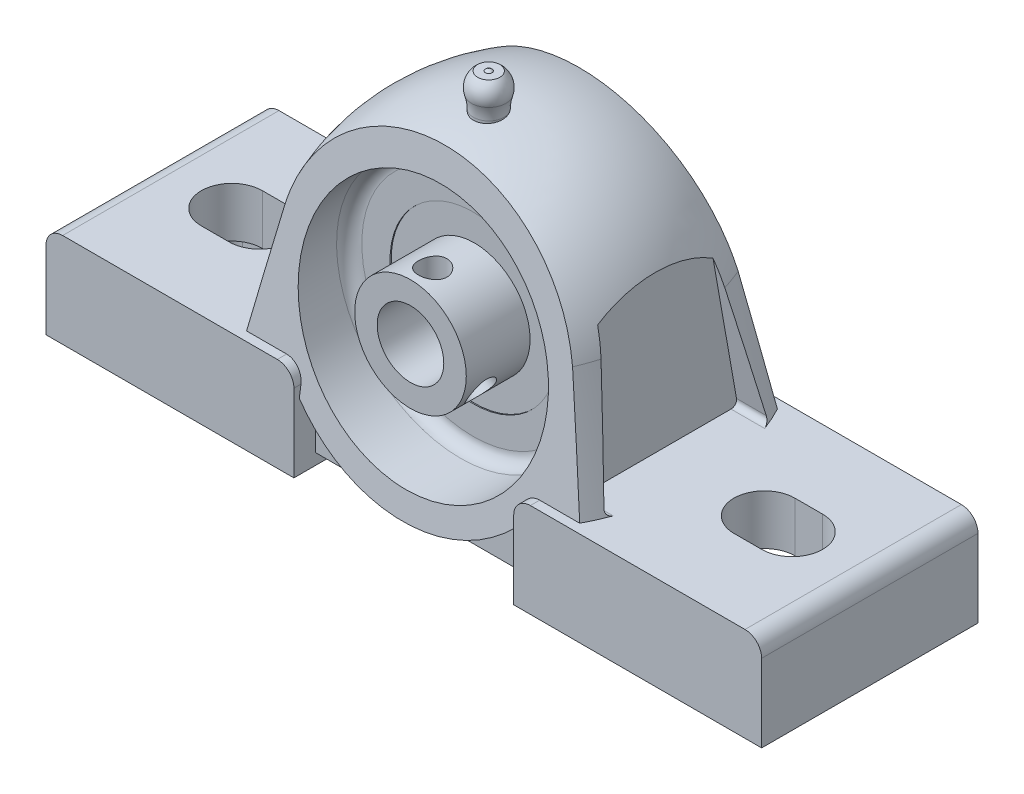
from build123d import *

# Parameters (mm, degrees)
BASE_EXTRUDE_DEPTH              = 78.25
CUT_EXTRUDE1_DEPTH              = 53.051467171
CUT_EXTRUDE1_DEPTH_BACK         = 53.051467171
SKETCH5_OUTSIDE_W               = 59.682
SKETCH5_OUTSIDE_H               = 80.692
BOSS_EXTRUDE4_REACH             = 57.711
BOSS_EXTRUDE4_DIRECTION_2_REACH = 57.711
BOSS_EXTRUDE1_DEPTH             = 19.5
BOSS_EXTRUDE1_DEPTH_BACK        = 19.5
CUT_EXTRUDE3_DEPTH              = 95.411036953
CUT_EXTRUDE4_DEPTH              = 7.99
CUT_EXTRUDE4_DRAFT              = -1
CUT_EXTRUDE4_PROFILE_2_DEPTH    = 7.99
CUT_EXTRUDE4_PROFILE_2_DRAFT    = -1
CIRPATTERN1_COUNT               = 9
SKETCH14_W                      = 31
SKETCH14_H                      = 4.06
SKETCH16_W                      = 2.567
SKETCH16_H                      = 6.26
SKETCH15_W                      = 0.1
SKETCH15_H                      = 5.32
CIRPATTERN2_COUNT               = 2
CIRPATTERN2_ANGLE               = 120
CUT_EXTRUDE5_START              = 25.83943
CUT_EXTRUDE5_DEPTH              = 12.56057
CUT_EXTRUDE6_START              = -38.4
CUT_EXTRUDE6_DEPTH              = 12.24096


with BuildPart() as part:
    # Sketch1 → Base-Extrude (new body)
    with BuildSketch(Plane(origin=(0, -28.2, 0), x_dir=(-1, 0, 0), z_dir=(0, 1, 0))):
        with BuildLine():
            Line((-33.636057661, 18.525), (33.636057661, 18.525))
            ThreePointArc((33.636057661, 18.525), (38.4, 0), (33.636057661, -18.525))
            Line((33.636057661, -18.525), (-33.636057661, -18.525))
            ThreePointArc((-33.636057661, -18.525), (-38.4, 0), (-33.636057661, 18.525))
        make_face()
    extrude(amount=BASE_EXTRUDE_DEPTH)

    # Cut-Sweep1: sweep along a path in Sketch3
    with BuildLine(Plane.XY) as cut_sweep1_path:
        Line((-38.4, -28.2), (-28.856466036, 7.676194886))
        ThreePointArc((-28.856466036, 7.676194886), (0, 29.86), (28.856466036, 7.676194886))
        Line((28.856466036, 7.676194886), (38.4, -28.2))
    # Sketch2 → Cut-Sweep1 (sweep, cut)
    with BuildSketch(Plane(origin=(0, -28.2, 0), x_dir=(-1, 0, 0), z_dir=(0, 1, 0))):
        with BuildLine():
            Line((-33.636057661, 18.525), (-116.65, 18.525))
            Line((-116.65, 18.525), (-116.65, -18.525))
            Line((-116.65, -18.525), (-33.636057661, -18.525))
            ThreePointArc((-33.636057661, -18.525), (-38.4, 0), (-33.636057661, 18.525))
        make_face()
    sweep(path=cut_sweep1_path.line, mode=Mode.SUBTRACT)

    # Sketch5 outside → Cut-Extrude1 (cut, two sides: drawn at the far end of the back side and taken through both)
    with BuildSketch(Plane(origin=(0, 0, 0), x_dir=(0, 0, -1), z_dir=(1, 0, 0)).offset(-CUT_EXTRUDE1_DEPTH_BACK)):
        with Locations((0, 0.83)):
            Rectangle(SKETCH5_OUTSIDE_W, SKETCH5_OUTSIDE_H)
        Polygon((11.7, 30.86), (18.525, -18.28), (15.6, -18.28), (15.6, -31.2), (-15.6, -31.2), (-15.6, -18.28), (-18.525, -18.28), (-11.7, 30.86), align=None, mode=Mode.SUBTRACT)
    extrude(amount=CUT_EXTRUDE1_DEPTH + CUT_EXTRUDE1_DEPTH_BACK, mode=Mode.SUBTRACT)

    # Sketch6 → Cut-Revolve2 (revolve, cut)
    with BuildSketch(Plane(origin=(0, 0, 0), x_dir=(0, 0, -1), z_dir=(1, 0, 0)), mode=Mode.PRIVATE) as cut_revolve2_sk:
        with BuildLine():
            Line((-22.725865299, 22.347619048), (-9.277190476, 22.347619048))
            ThreePointArc((-9.277190476, 22.347619048), (-7.666973648, 21.680645399), (-7, 20.070428571))
            Line((-7, 20.070428571), (-7, 18.734993995))
            ThreePointArc((-7, 18.734993995), (-6.071328156, 19.056205667), (-5.128, 19.331415261))
            Line((-5.128, 19.331415261), (-5.128, 22.347619048))
            Line((-5.128, 22.347619048), (-3.256, 22.347619048))
            Line((-3.256, 22.347619048), (-3.256, 19.733181801))
            ThreePointArc((-3.256, 19.733181801), (1.937389668, 19.905941859), (7, 18.734993995))
            Line((7, 18.734993995), (7, 20.070428571))
            ThreePointArc((7, 20.070428571), (7.666973648, 21.680645399), (9.277190476, 22.347619048))
            Line((9.277190476, 22.347619048), (22.725865299, 22.347619048))
            Line((22.725865299, 22.347619048), (25.829701277, 0))
            Line((25.829701277, 0), (-25.829701277, 0))
            Line((-25.829701277, 0), (-22.725865299, 22.347619048))
        make_face()
    revolve(cut_revolve2_sk.sketch.rotate(Axis((0, 0, 0), (0, 0, -1)), 180), axis=Axis((0, 0, 0), (0, 0, -1)), mode=Mode.SUBTRACT)

    # Sketch11 → Boss-Revolve1 (revolve)
    with BuildSketch(Plane.XY.offset(4.192)):
        with BuildLine():
            Line((0, 27.973774284), (0, 35.86))
            ThreePointArc((0, 35.86), (-0.328456711, 35.790107141), (-0.6, 35.592539267))
            Line((-0.6, 35.592539267), (-2, 35.592539267))
            ThreePointArc((-2, 35.592539267), (-3.100653507, 34.004684437), (-3.105555556, 32.072665525))
            ThreePointArc((-3.105555556, 32.072665525), (-2.83938828, 30.906746373), (-2.75, 29.714176785))
            Line((-2.75, 29.714176785), (-2.75, 27.973774284))
            Line((-2.75, 27.973774284), (0, 27.973774284))
        make_face()
    revolve(axis=Axis((0, 0, 4.192), (0, 1, 0)))

    # Boss-Extrude4: up to this plane
    boss_extrude4_end = Plane(origin=(-38.4, 30.86, -11.7), z_dir=(0, 0.137568371274657, -0.9904922731777558))
    # Sketch9 → Boss-Extrude4 (add, up to the surface)
    with BuildSketch(Plane.XY, mode=Mode.PRIVATE) as boss_extrude4_sk1:
        with BuildLine():
            Line((12.855258733, -18.28), (19.810146566, -18.28))
            ThreePointArc((19.810146566, -18.28), (0, -26.955524609), (-19.810146566, -18.28))
            Line((-19.810146566, -18.28), (-12.855258733, -18.28))
            ThreePointArc((-12.855258733, -18.28), (0, -22.347619048), (12.855258733, -18.28))
        make_face()
    boss_extrude4_tool1 = split(extrude(boss_extrude4_sk1.sketch, amount=-BOSS_EXTRUDE4_REACH, mode=Mode.PRIVATE), bisect_by=boss_extrude4_end, keep=Keep.BOTH, mode=Mode.PRIVATE)
    add(boss_extrude4_tool1.solids().sort_by_distance((0, -22.606339, 0))[0])

    # Boss-Extrude4 direction 2: up to this plane
    boss_extrude4_direction_2_end = Plane(origin=(-38.4, 30.86, 11.7), z_dir=(0, 0.137568371274657, 0.9904922731777558))
    # Sketch9 → Boss-Extrude4 direction 2 (add, up to the surface)
    with BuildSketch(Plane.XY, mode=Mode.PRIVATE) as boss_extrude4_direction_2_sk1:
        with BuildLine():
            Line((12.855258733, -18.28), (19.810146566, -18.28))
            ThreePointArc((19.810146566, -18.28), (0, -26.955524609), (-19.810146566, -18.28))
            Line((-19.810146566, -18.28), (-12.855258733, -18.28))
            ThreePointArc((-12.855258733, -18.28), (0, -22.347619048), (12.855258733, -18.28))
        make_face()
    boss_extrude4_direction_2_tool1 = split(extrude(boss_extrude4_direction_2_sk1.sketch, amount=BOSS_EXTRUDE4_DIRECTION_2_REACH, mode=Mode.PRIVATE), bisect_by=boss_extrude4_direction_2_end, keep=Keep.BOTH, mode=Mode.PRIVATE)
    add(boss_extrude4_direction_2_tool1.solids().sort_by_distance((0, -22.606339, 0))[0])

    # Sketch4 → Boss-Extrude1 (add, two sides: drawn at the far end of the back side and taken through both)
    with BuildSketch(Plane.XY.offset(-BOSS_EXTRUDE1_DEPTH_BACK)):
        with BuildLine():
            Line((22.810146566, -13.2), (61.5, -13.2))
            ThreePointArc((61.5, -13.2), (63.621320344, -14.078679656), (64.5, -16.2))
            Line((64.5, -16.2), (64.5, -30.2))
            Line((64.5, -30.2), (19.810146566, -30.2))
            Line((19.810146566, -30.2), (19.810146566, -16.2))
            ThreePointArc((19.810146566, -16.2), (20.688826222, -14.078679656), (22.810146566, -13.2))
        make_face()
        with BuildLine():
            Line((-61.5, -13.2), (-22.810146566, -13.2))
            ThreePointArc((-22.810146566, -13.2), (-20.688826222, -14.078679656), (-19.810146566, -16.2))
            Line((-19.810146566, -16.2), (-19.810146566, -30.2))
            Line((-19.810146566, -30.2), (-64.5, -30.2))
            Line((-64.5, -30.2), (-64.5, -16.2))
            ThreePointArc((-64.5, -16.2), (-63.621320344, -14.078679656), (-61.5, -13.2))
        make_face()
    extrude(amount=BOSS_EXTRUDE1_DEPTH + BOSS_EXTRUDE1_DEPTH_BACK)

    # Sketch7 → Cut-Extrude3 (cut, through all)
    with BuildSketch(Plane.XZ.offset(30.2)):
        with BuildLine():
            Line((-45.5, 5.5), (-50.5, 5.5))
            ThreePointArc((-50.5, 5.5), (-56, 0), (-50.5, -5.5))
            Line((-50.5, -5.5), (-45.5, -5.5))
            ThreePointArc((-45.5, -5.5), (-40, 0), (-45.5, 5.5))
        make_face()
        with BuildLine():
            Line((45.5, -5.5), (50.5, -5.5))
            ThreePointArc((50.5, -5.5), (56, 0), (50.5, 5.5))
            Line((50.5, 5.5), (45.5, 5.5))
            ThreePointArc((45.5, 5.5), (40, 0), (45.5, -5.5))
        make_face()
    extrude(amount=-CUT_EXTRUDE3_DEPTH, mode=Mode.SUBTRACT)


with BuildPart() as cut_extrude4_tool:
    # Sketch10 → Cut-Extrude4 (with draft: the straight prism first)
    with BuildSketch(Plane.XZ.offset(30.2)):
        with BuildLine():
            ThreePointArc((50.5, -10.73), (51.015492065, -9.485492065), (52.26, -8.97))
            Line((52.26, -8.97), (57.475, -8.97))
            ThreePointArc((57.475, -8.97), (58.719507935, -8.454507935), (59.235, -7.21))
            Line((59.235, -7.21), (59.235, 7.21))
            ThreePointArc((59.235, 7.21), (58.719507935, 8.454507935), (57.475, 8.97))
            Line((57.475, 8.97), (52.26, 8.97))
            ThreePointArc((52.26, 8.97), (51.015492065, 9.485492065), (50.5, 10.73))
            Line((50.5, 10.73), (50.5, 12.475))
            ThreePointArc((50.5, 12.475), (49.984507935, 13.719507935), (48.74, 14.235))
            Line((48.74, 14.235), (26.835146566, 14.235))
            ThreePointArc((26.835146566, 14.235), (25.590638631, 13.719507935), (25.075146566, 12.475))
            Line((25.075146566, 12.475), (25.075146566, -12.475))
            ThreePointArc((25.075146566, -12.475), (25.590638631, -13.719507935), (26.835146566, -14.235))
            Line((26.835146566, -14.235), (48.74, -14.235))
            ThreePointArc((48.74, -14.235), (49.984507935, -13.719507935), (50.5, -12.475))
            Line((50.5, -12.475), (50.5, -10.73))
        make_face()
    extrude(amount=-CUT_EXTRUDE4_DEPTH)
    # Cut-Extrude4: the draft: its side faces are tilted about the plane it starts from
    cut_extrude4_sides = [cut_extrude4_tool.faces().sort_by_distance(p)[0] for p in [
        (51.015492065, -26.205, -9.485492065),
        (54.8675, -26.205, -8.97),
        (58.719507935, -26.205, -8.454507935),
        (59.235, -26.205, 0),
        (58.719507935, -26.205, 8.454507935),
        (54.8675, -26.205, 8.97),
        (51.015492065, -26.205, 9.485492065),
        (50.5, -26.205, 11.6025),
        (49.984507935, -26.205, 13.719507935),
        (37.787573283, -26.205, 14.235),
        (25.590638631, -26.205, 13.719507935),
        (25.075146566, -26.205, 0),
        (25.590638631, -26.205, -13.719507935),
        (37.787573283, -26.205, -14.235),
        (49.984507935, -26.205, -13.719507935),
        (50.5, -26.205, -11.6025),
    ]]
    draft(cut_extrude4_sides, Plane.XZ.offset(30.2), CUT_EXTRUDE4_DRAFT)


with BuildPart() as part_1:
    add(part.part)

    # Cut-Extrude4: cut by cut_extrude4_tool
    add(cut_extrude4_tool.part, mode=Mode.SUBTRACT)


with BuildPart() as cut_extrude4_profile_2_tool:
    # Sketch10 → Cut-Extrude4 profile 2 (with draft: the straight prism first)
    with BuildSketch(Plane.XZ.offset(30.2)):
        with BuildLine():
            Line((-57.475, -8.97), (-52.26, -8.97))
            ThreePointArc((-52.26, -8.97), (-51.015492065, -9.485492065), (-50.5, -10.73))
            Line((-50.5, -10.73), (-50.5, -12.475))
            ThreePointArc((-50.5, -12.475), (-49.984507935, -13.719507935), (-48.74, -14.235))
            Line((-48.74, -14.235), (-26.835146566, -14.235))
            ThreePointArc((-26.835146566, -14.235), (-25.590638631, -13.719507935), (-25.075146566, -12.475))
            Line((-25.075146566, -12.475), (-25.075146566, 12.475))
            ThreePointArc((-25.075146566, 12.475), (-25.590638631, 13.719507935), (-26.835146566, 14.235))
            Line((-26.835146566, 14.235), (-48.74, 14.235))
            ThreePointArc((-48.74, 14.235), (-49.984507935, 13.719507935), (-50.5, 12.475))
            Line((-50.5, 12.475), (-50.5, 10.73))
            ThreePointArc((-50.5, 10.73), (-51.015492065, 9.485492065), (-52.26, 8.97))
            Line((-52.26, 8.97), (-57.475, 8.97))
            ThreePointArc((-57.475, 8.97), (-58.719507935, 8.454507935), (-59.235, 7.21))
            Line((-59.235, 7.21), (-59.235, -7.21))
            ThreePointArc((-59.235, -7.21), (-58.719507935, -8.454507935), (-57.475, -8.97))
        make_face()
    extrude(amount=-CUT_EXTRUDE4_PROFILE_2_DEPTH)
    # Cut-Extrude4 profile 2: the draft: its side faces are tilted about the plane it starts from
    cut_extrude4_profile_2_sides = [cut_extrude4_profile_2_tool.faces().sort_by_distance(p)[0] for p in [
        (-58.719507935, -26.205, 8.454507935),
        (-59.235, -26.205, 0),
        (-58.719507935, -26.205, -8.454507935),
        (-54.8675, -26.205, -8.97),
        (-51.015492065, -26.205, -9.485492065),
        (-50.5, -26.205, -11.6025),
        (-49.984507935, -26.205, -13.719507935),
        (-37.787573283, -26.205, -14.235),
        (-25.590638631, -26.205, -13.719507935),
        (-25.075146566, -26.205, 0),
        (-25.590638631, -26.205, 13.719507935),
        (-37.787573283, -26.205, 14.235),
        (-49.984507935, -26.205, 13.719507935),
        (-50.5, -26.205, 11.6025),
        (-51.015492065, -26.205, 9.485492065),
        (-54.8675, -26.205, 8.97),
    ]]
    draft(cut_extrude4_profile_2_sides, Plane.XZ.offset(30.2), CUT_EXTRUDE4_PROFILE_2_DRAFT)


with BuildPart() as part_2:
    add(part_1.part)

    # Cut-Extrude4 profile 2: cut by cut_extrude4_profile_2_tool
    add(cut_extrude4_profile_2_tool.part, mode=Mode.SUBTRACT)

    # Sketch12 → Boss-Revolve3 (revolve)
    with BuildSketch(Plane(origin=(0, 0, 0), x_dir=(0, 0, -1), z_dir=(1, 0, 0)), mode=Mode.PRIVATE) as boss_revolve3_sk:
        with BuildLine():
            Line((7, 18.754993995), (7, 14.98))
            Line((7, 14.98), (-7, 14.98))
            Line((-7, 14.98), (-7, 18.754993995))
            ThreePointArc((-7, 18.754993995), (0, 20.02), (7, 18.754993995))
        make_face()
    revolve(boss_revolve3_sk.sketch.rotate(Axis((0, 0, 0), (0, 0, -1)), 180), axis=Axis((0, 0, 0), (0, 0, -1)))

    # Sketch13 → Boss-Revolve4 (revolve)
    with BuildSketch(Plane(origin=(0, 0, 0), x_dir=(0, 0, -1), z_dir=(1, 0, 0))):
        with BuildLine():
            Line((0, 17.01), (0, 9.03))
            ThreePointArc((0, 9.03), (3.99, 13.02), (0, 17.01))
        make_face()
    boss_revolve4 = revolve(axis=Axis((0, 0, 0), (0, 1, 0)))

    # CirPattern1: Boss-Revolve4 ×9 about axis
    cirpattern1_axis = Axis((0, 0, 0), (0, 0, 1))
    for i in range(1, CIRPATTERN1_COUNT):
        add(boss_revolve4.rotate(cirpattern1_axis, i * 360 / CIRPATTERN1_COUNT))

    # Sketch14 → Boss-Revolve5 (revolve)
    with BuildSketch(Plane(origin=(0, 0, 0), x_dir=(0, 0, -1), z_dir=(1, 0, 0)), mode=Mode.PRIVATE) as boss_revolve5_sk:
        with Locations((-2.8, 8.03)):
            Rectangle(SKETCH14_W, SKETCH14_H)
    revolve(boss_revolve5_sk.sketch.rotate(Axis((0, 0, 0), (0, 0, -1)), 90), axis=Axis((0, 0, 0), (0, 0, -1)))

    # Sketch16 → Cut-Revolve3 (revolve, cut)
    with BuildSketch(Plane(origin=(0, 0, 0), x_dir=(0, 0, -1), z_dir=(1, 0, 0))):
        with Locations((-15.5835, 7.13)):
            Rectangle(SKETCH16_W, SKETCH16_H)
    cut_revolve3 = revolve(axis=Axis((0, 10.26, 14.3), (0, -1, 0)), mode=Mode.SUBTRACT)

    # Sketch15 → Boss-Revolve6 (revolve)
    with BuildSketch(Plane(origin=(0, 0, 0), x_dir=(0, 0, -1), z_dir=(1, 0, 0)), mode=Mode.PRIVATE) as boss_revolve6_sk:
        with Locations((-6.75, 12.52)):
            Rectangle(SKETCH15_W, SKETCH15_H)
        with Locations((6.75, 12.52)):
            Rectangle(SKETCH15_W, SKETCH15_H)
    revolve(boss_revolve6_sk.sketch.rotate(Axis((0, 0, 0), (0, 0, -1)), 90), axis=Axis((0, 0, 0), (0, 0, -1)))

    # CirPattern2: Cut-Revolve3 ×2 about axis
    cirpattern2_axis = Axis((0, 0, -21.702927371), (0, 0, -1))
    for i in range(1, CIRPATTERN2_COUNT):
        add(cut_revolve3.rotate(cirpattern2_axis, i * CIRPATTERN2_ANGLE / (CIRPATTERN2_COUNT - 1)), mode=Mode.SUBTRACT)

    # Sketch 17_2 → Cut-Extrude5 (cut)
    with BuildSketch(Plane(origin=(0, 0, 0), x_dir=(0, 0, -1), z_dir=(1, 0, 0)).offset(CUT_EXTRUDE5_START)):
        with BuildLine():
            Line((7.573865879, 27.973774284), (-7.573865879, 27.973774284))
            Line((-7.573865879, 27.973774284), (-14.626967343, -12.026351822))
            ThreePointArc((-14.626967343, -12.026351822), (-14.408204033, -12.84278761), (-13.64215959, -13.2))
            Line((-13.64215959, -13.2), (13.64215959, -13.2))
            ThreePointArc((13.64215959, -13.2), (14.408204033, -12.84278761), (14.626967343, -12.026351822))
            Line((14.626967343, -12.026351822), (7.573865879, 27.973774284))
        make_face()
    extrude(amount=CUT_EXTRUDE5_DEPTH, mode=Mode.SUBTRACT)

    # Sketch 17_2 2 → Cut-Extrude6 (cut)
    with BuildSketch(Plane(origin=(0, 0, 0), x_dir=(0, 0, -1), z_dir=(1, 0, 0)).offset(CUT_EXTRUDE6_START)):
        with BuildLine():
            Line((7.573865879, 27.973774284), (-7.573865879, 27.973774284))
            Line((-7.573865879, 27.973774284), (-14.626967343, -12.026351822))
            ThreePointArc((-14.626967343, -12.026351822), (-14.408204033, -12.84278761), (-13.64215959, -13.2))
            Line((-13.64215959, -13.2), (13.64215959, -13.2))
            ThreePointArc((13.64215959, -13.2), (14.408204033, -12.84278761), (14.626967343, -12.026351822))
            Line((14.626967343, -12.026351822), (7.573865879, 27.973774284))
        make_face()
    extrude(amount=CUT_EXTRUDE6_DEPTH, mode=Mode.SUBTRACT)


solid = part_2.part
